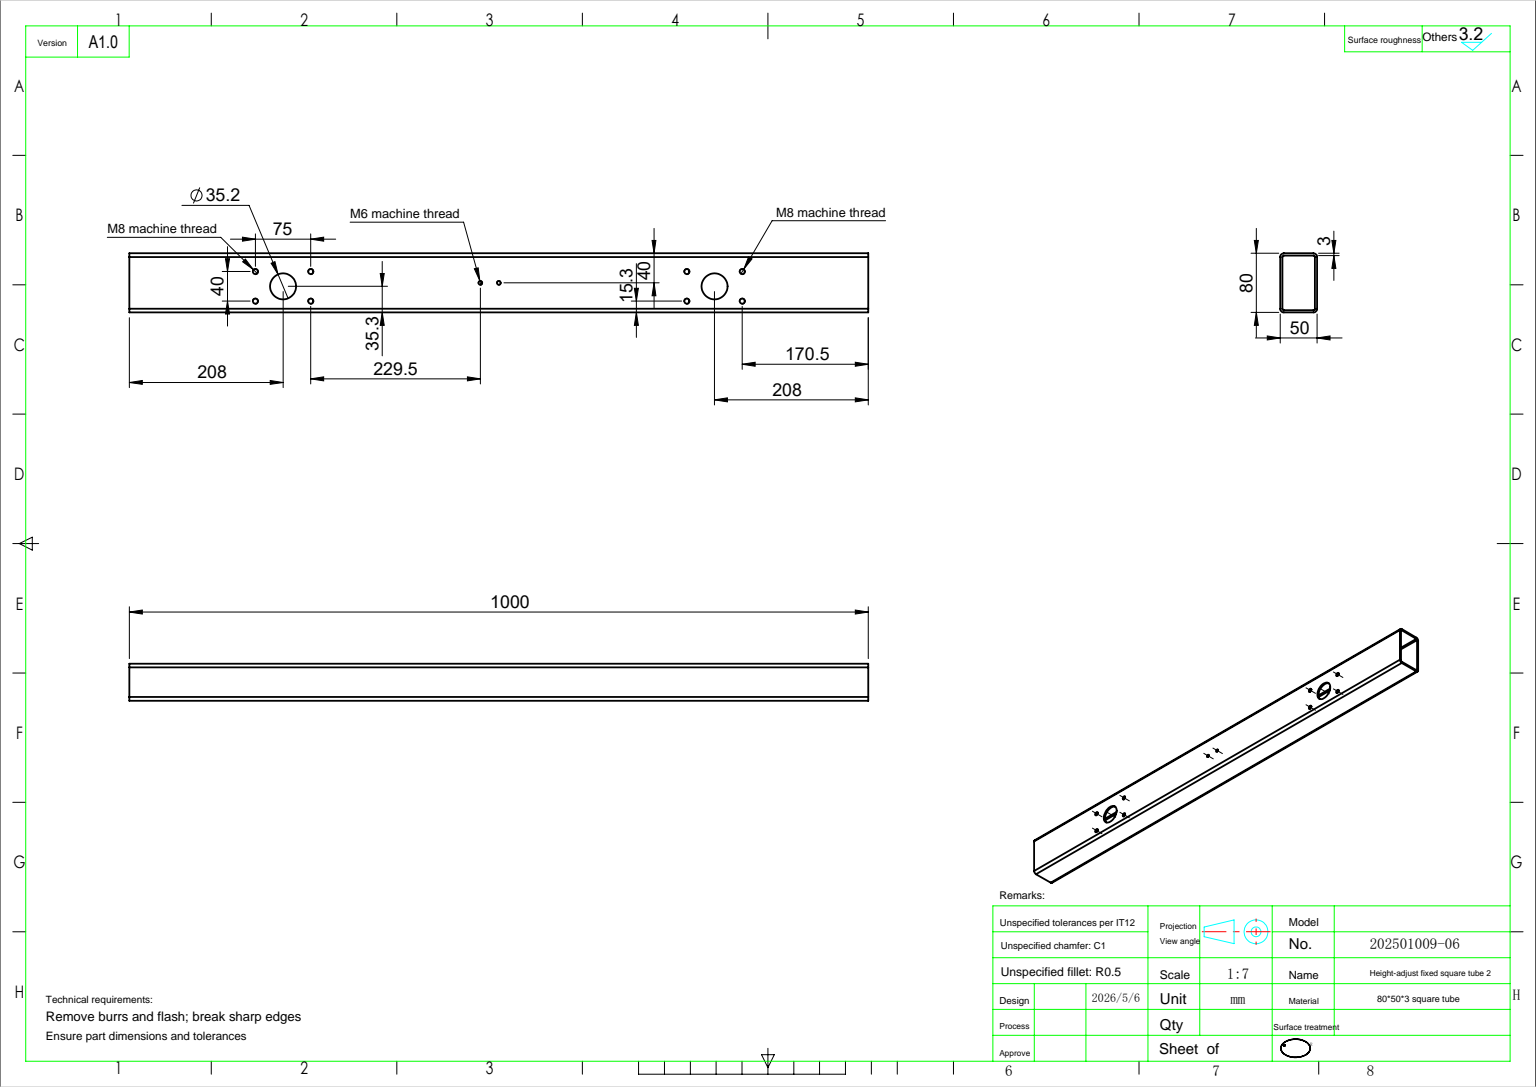
from build123d import *

# Parameters (mm, degrees)
SKETCH_1_W          = 80
SKETCH_1_H          = 50
EXTRUDE_1_DEPTH     = 1000
FILLET_1_R          = 5
SHELL_1_T           = -3
SKETCH_2_R          = 17.6
CUT_EXTRUDE_1_DEPTH = 1003.047903047
SKETCH_3_R          = 3.4
CUT_EXTRUDE_2_DEPTH = 10
SKETCH_4_R          = 2.5
CUT_EXTRUDE_3_DEPTH = 10


with BuildPart() as part:
    # 草图1 → 凸台-拉伸1 (new body)
    with BuildSketch(Plane.XY):
        Rectangle(SKETCH_1_W, SKETCH_1_H)
    extrude(amount=EXTRUDE_1_DEPTH)

    # 圆角1
    fillet_1_edges = [part.edges().sort_by_distance(p)[0] for p in [
        (40, -25, 500),
        (-40, -25, 500),
        (-40, 25, 500),
        (40, 25, 500),
    ]]
    fillet(fillet_1_edges, radius=FILLET_1_R)

    # 抽壳1
    shell_1_openings = [part.faces().sort_by_distance(p)[0] for p in [
        (0, 0, 1000),
        (0, 0, 0),
    ]]
    offset(amount=SHELL_1_T, openings=shell_1_openings, kind=Kind.INTERSECTION)

    # 草图2 → 切除-拉伸1 (cut, through all)
    with BuildSketch(Plane(origin=(0, 25, 0), x_dir=(1, 0, 0), z_dir=(0, 1, 0))):
        with Locations(Location((-4.7, -208, 0), (0, 0, 270))):
            Circle(SKETCH_2_R)
        with Locations(Location((-4.7, -792, 0), (0, 0, 270))):
            Circle(SKETCH_2_R)
    extrude(amount=-CUT_EXTRUDE_1_DEPTH, mode=Mode.SUBTRACT)

    # 草图3 → 切除-拉伸2 (cut)
    with BuildSketch(Plane(origin=(0, 25, 0), x_dir=(1, 0, 0), z_dir=(0, 1, 0))):
        with Locations(Location((15.3, -170.5, 0), (0, 0, 270))):
            Circle(SKETCH_3_R)
        with Locations(Location((-24.7, -170.5, 0), (0, 0, 270))):
            Circle(SKETCH_3_R)
        with Locations(Location((-24.7, -245.5, 0), (0, 0, 270))):
            Circle(SKETCH_3_R)
        with Locations(Location((15.3, -245.5, 0), (0, 0, 270))):
            Circle(SKETCH_3_R)
        with Locations(Location((15.3, -754.5, 0), (0, 0, 270))):
            Circle(SKETCH_3_R)
        with Locations(Location((-24.7, -754.5, 0), (0, 0, 270))):
            Circle(SKETCH_3_R)
        with Locations(Location((-24.7, -829.5, 0), (0, 0, 270))):
            Circle(SKETCH_3_R)
        with Locations(Location((15.3, -829.5, 0), (0, 0, 270))):
            Circle(SKETCH_3_R)
    extrude(amount=-CUT_EXTRUDE_2_DEPTH, mode=Mode.SUBTRACT)

    # 草图4 → 切除-拉伸3 (cut)
    with BuildSketch(Plane(origin=(0, 25, 0), x_dir=(1, 0, 0), z_dir=(0, 1, 0))):
        with Locations(Location((0, -475, 0), (0, 0, 270))):
            Circle(SKETCH_4_R)
        with Locations(Location((0, -500, 0), (0, 0, 270))):
            Circle(SKETCH_4_R)
    extrude(amount=-CUT_EXTRUDE_3_DEPTH, mode=Mode.SUBTRACT)


solid = part.part
